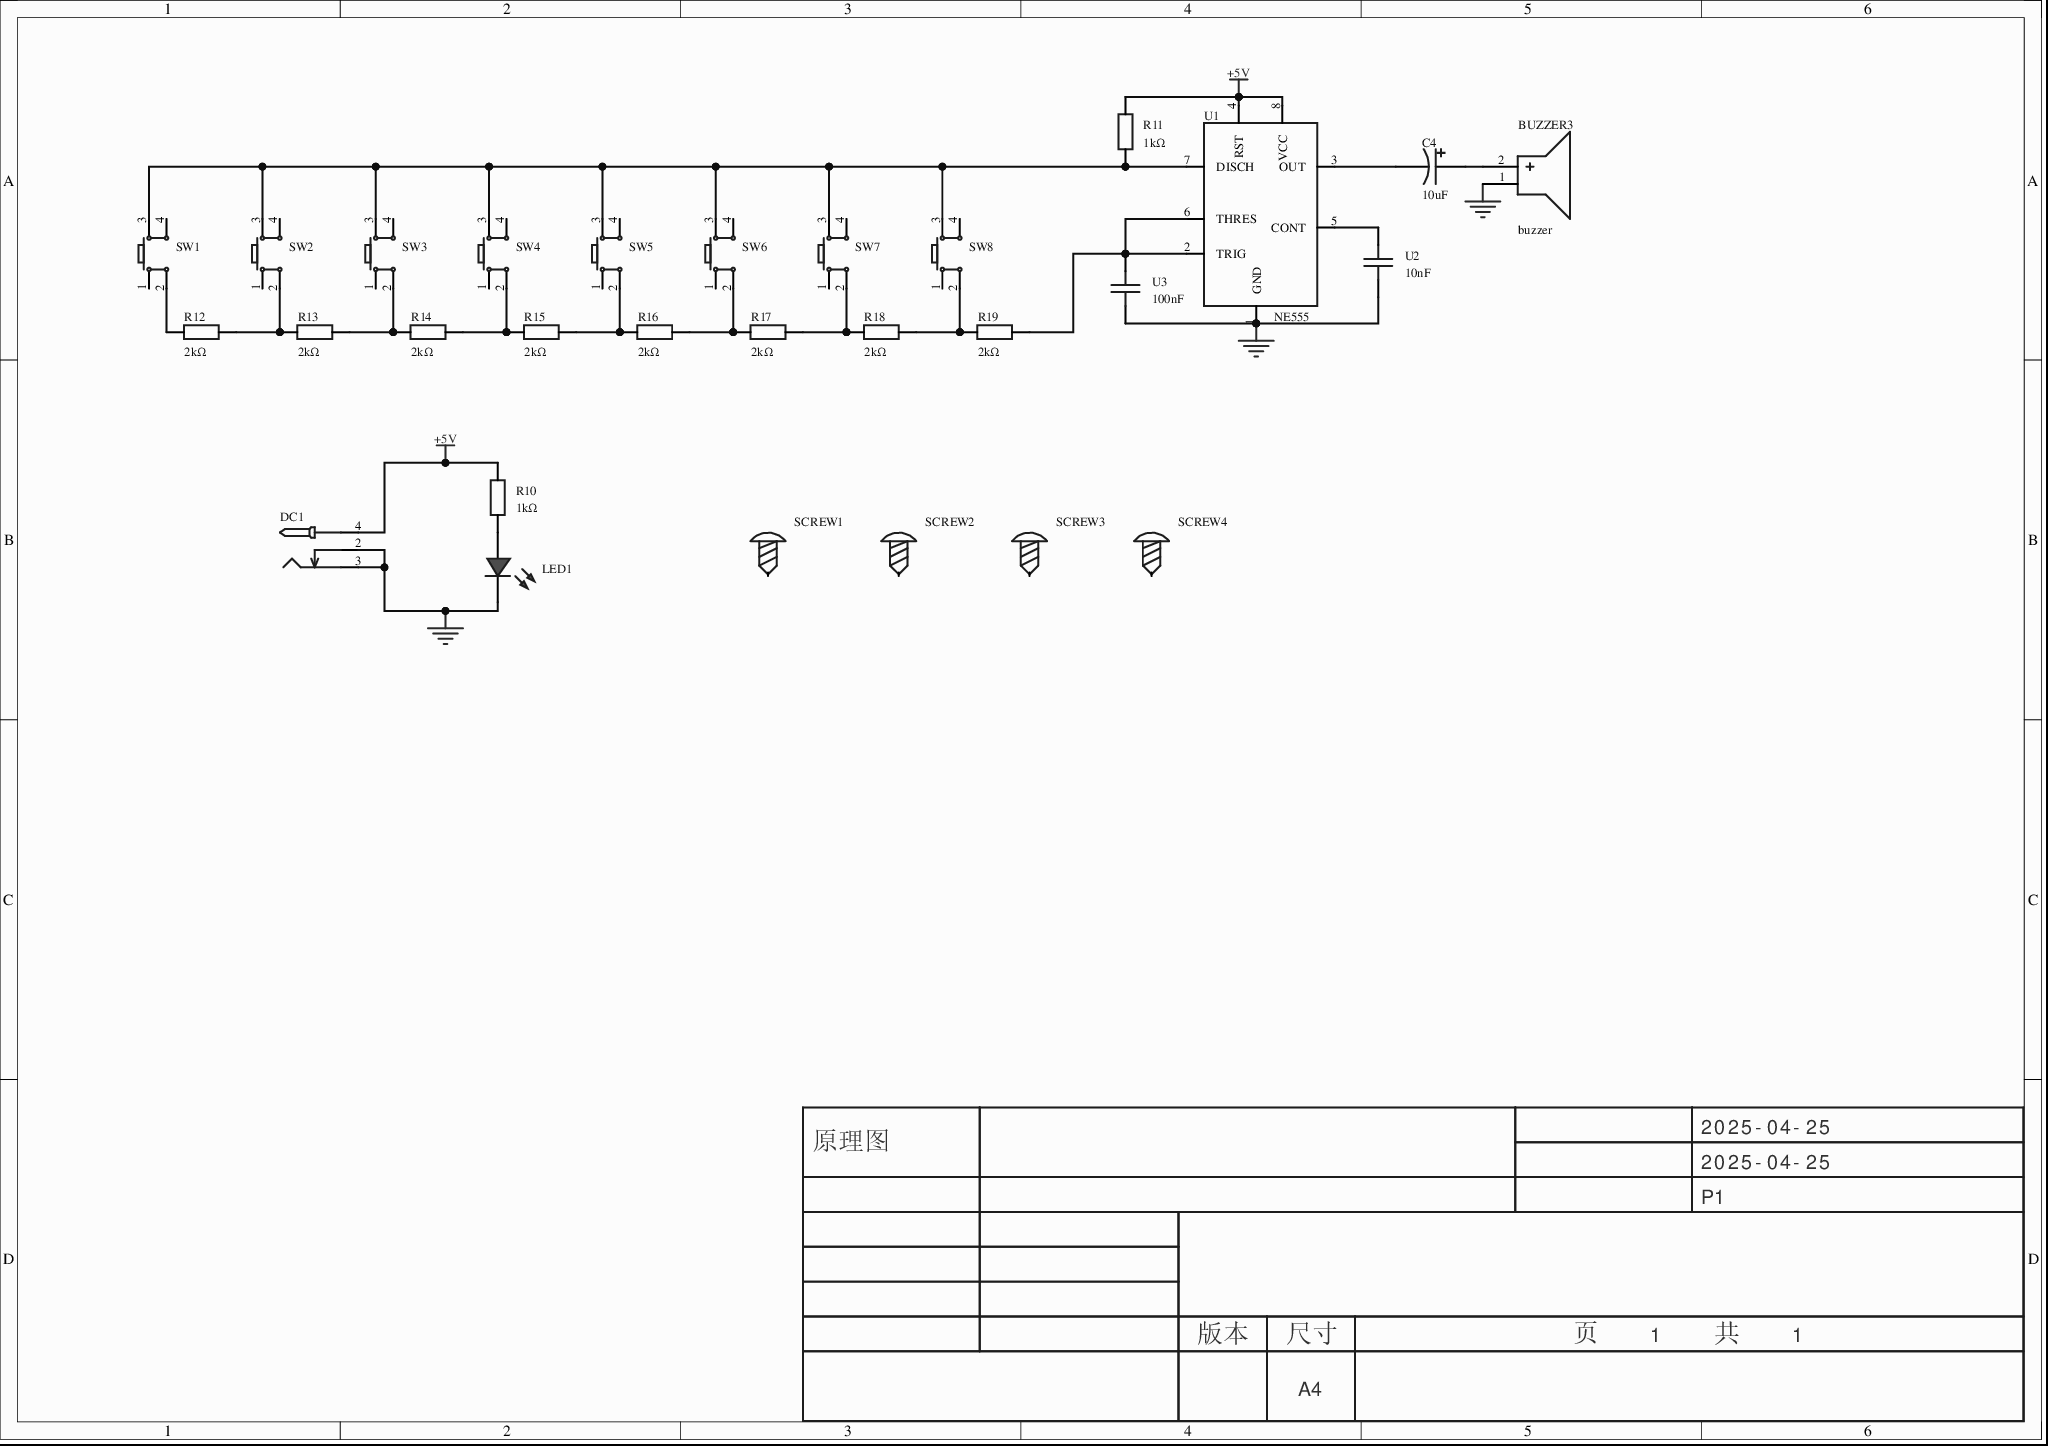
[diagram p0: MISC52051-3.schdoc]
# Altium project MISC52051-2.PrjPcb
1 sheet, 29 parts. Net scope: global (net labels, ports and power ports of the same name join across sheets).
Board file: MISC52051.pcbdoc

## Sheet MISC52051-3.schdoc
size 297 x 209 mm; Version: V1.0; @Project Name: MISC52051; @Page Count: 1; @Update Date: 2025-04-25; @Create Date: 2025-04-25; @Schematic Name: MISC52051; @Page No: 1; @Create Time: 16:50:07; @Update Time: 17:02:59; @Board Name: MISC52051

### Parts
BUZZER3  buzzer  [BUZ-TH_BD12.0-P6.00-D0.9-RD]
C4  10uF  [CAP-TH_BD5.0-P2.00-D0.8-FD]
DC1  (no value)  [DC-2.0]
LED1  (no value)  [LED_TH-3mm]
R10  1kΩ  [Res_1/8W]
R11  1kΩ  [Res_1/8W]
R12  2kΩ  [Res_1/8W]
R13  2kΩ  [Res_1/8W]
R14  2kΩ  [Res_1/8W]
R15  2kΩ  [Res_1/8W]
R16  2kΩ  [Res_1/8W]
R17  2kΩ  [Res_1/8W]
R18  2kΩ  [Res_1/8W]
R19  2kΩ  [Res_1/8W]
SCREW1  (no value)  [M3螺丝]
SCREW2  (no value)  [M3螺丝]
SCREW3  (no value)  [M3螺丝]
SCREW4  (no value)  [M3螺丝]
SW1  (no value)  [SW-TH_4P-L6.0-W6.0-P4.50-LS6.5]
SW2  (no value)  [SW-TH_4P-L6.0-W6.0-P4.50-LS6.5]
SW3  (no value)  [SW-TH_4P-L6.0-W6.0-P4.50-LS6.5]
SW4  (no value)  [SW-TH_4P-L6.0-W6.0-P4.50-LS6.5]
SW5  (no value)  [SW-TH_4P-L6.0-W6.0-P4.50-LS6.5]
SW6  (no value)  [SW-TH_4P-L6.0-W6.0-P4.50-LS6.5]
SW7  (no value)  [SW-TH_4P-L6.0-W6.0-P4.50-LS6.5]
SW8  (no value)  [SW-TH_4P-L6.0-W6.0-P4.50-LS6.5]
U1  NE555  [PDIP-8_L9.6-W6.4-P2.54-LS7.9-BL-1]
U2  10nF  [CAP-TH_L4.0-W2.5-P2.50-D0.5]
U3  100nF  [CAP-TH_L4.0-W2.5-P2.50-D0.5]

### Nets
+5V: DC1.4 R10.2 R11.2 U1.4(RST) U1.8(VCC)
GND: BUZZER3.1(-) DC1.2 DC1.3 LED1.2(A) U1.1(GND) U2.1 U3.1
NetBUZZER3_2: BUZZER3.2(+) C4.1
NetC4_2: C4.2 U1.3(OUT)
NetLED1_1: LED1.1(C) R10.1
NetR11_1: R11.1 SW1.3 SW2.3 SW3.3 SW4.3 SW5.3 SW6.3 SW7.3 SW8.3 U1.7(DISCH)
NetR12_1: R12.1 SW1.2
NetR12_2: R12.2 R13.1 SW2.2
NetR13_2: R13.2 R14.1 SW3.2
NetR14_2: R14.2 R15.1 SW4.2
NetR15_2: R15.2 R16.1 SW5.2
NetR16_2: R16.2 R17.1 SW6.2
NetR17_2: R17.2 R18.1 SW7.2
NetR18_2: R18.2 R19.1 SW8.2
NetR19_2: R19.2 U1.2(TRIG) U1.6(THRES) U3.2
NetU1_5: U1.5(CONT) U2.2

Not connected (* = marked no-connect by the designer): SCREW1 1; SCREW2 1; SCREW3 1; SCREW4 1; SW1 1 4; SW2 1 4; SW3 1 4; SW4 1 4; SW5 1 4; SW6 1 4; SW7 1 4; SW8 1 4

### Notes on the sheet
- 2025-04-25
- 原理图
- P1
- 版本
- 尺寸
- A4
- 页    1    共    1

### Library data of the parts
BUZZER3 = buzzer: AddInBom: yes; ModelId: af17e4151ed84fc2a628230bf2376363; ModelTransform: 472.44,472.176,0,270,0,0,0,0,-196.85; Symbol: BUZZER; Device: buzzer; LCSC Part Name: buzzer; SupplierPart: C9900014030; ManufacturerPart: buzzer; Supplier Footprint: buzzer; JLCPCB Part Class: 扩展库; Supplier: LCSC; ConvertToPcb: yes; FootprintName: BUZ-TH_BD12.0-P6.00-D0.9-RD; ModelName: BUZ-TH_BD12.0-P6.00-D0.9-RD
C4 = KM475M100D11RR0VH2FP0: 容值:4.7uF;精度:±20%;额定电压:100V;; Manufacturer: CX(承兴); Symbol: 4.7uF 100V 5*11; AddInBom: yes; ModelId: edeeed87cbc746108d01291548c38636; ModelName: CAP-TH_D5.0×H7.0×P2.0; ModelTransform: 197.091,196.7911,0,0,0,0,0,0,-137.795; Tolerance: ±20%; Rated Voltage: 100V; φD: 5mm; L: 11mm; Value: 10uF; Device: KM475M100D11RR0VH2FP0; LCSC Part Name: 4.7uF ±20% 100V; ManufacturerPart: KM475M100D11RR0VH2FP0; Supplier Footprint: 插件,D5xL11mm; JLCPCB Part Class: 扩展库; Datasheet: https://atta.szlcsc.com/upload/public/pdf/source/20211027/06D6BA3719C264B639DC286D935D03EA.pdf; Supplier: LCSC; ConvertToPcb: yes; FootprintName: CAP-TH_BD5.0-P2.00-D0.8-FD; Lead Spacing: 2mm; Lifetime @ Temp: -
DC1 = DC-005_2.0: ConvertToPcb: yes; SymbolName: DC电源接口; ModelId: f5f20b8a2308479b936ba3c2698865bb0819f05c4eef4c71ace90d822a990e87; ModelName: DC-IN-TH_DC-5520-1; ModelTransform: 372.05,551.18,582.68,90,0,0,137.8,0,-149.61; Device: DC-005_2.0; AddInBom: yes; Supplier Footprint: 插件; FootprintName: DC-2.0
LED1 = LED_TH-R_3mm: ConvertToPcb: yes; ModelId: a497c992633541038a38947cdc58012f; ModelName: LED-TH-3mm_R; ModelTransform: 141.274,153.327,0,0,0,0,-5.984,0,-137.795; Symbol: LED_TH-R; Device: LED_TH-R_3mm; AddInBom: yes; FootprintName: LED_TH-3mm; Supplier Footprint: 插件
R10-R19 = Res_AXIAL-1/8W: ConvertToPcb: yes; SymbolName: 电阻; ModelId: b2b5ae7ae4c642178fe0039925c86a3f; ModelName: RES-TH_BD1.8-L3.2-P7.20-D0.4; ModelTransform: 282.86,66.88,253.09,0,0,0,0,0,-191; Device: Res_AXIAL-1/8W; AddInBom: yes; Supplier Footprint: 轴向引线; FootprintName: Res_1/8W
  R10 R11: Value: 1kΩ
  R12-R19: Value: 2kΩ
SCREW1-SCREW4 = M3螺丝: ConvertToPcb: yes; SymbolName: 螺丝孔; Device: M3螺丝; AddInBom: yes; Supplier Footprint: 插件; FootprintName: M3螺丝
SW1-SW8 = Key_TH_6x6x6: 触点电流:50mA;额定电压(DC):12V;绝缘电阻:100MΩ;电路结构:单刀单掷;安装方式:直插;按钮形状:圆形按钮;按钮/盖帽颜色:黑色;作用力:260gf@±30gf;工作温度:-25℃~+70℃;引脚样式:PC引脚;开关长度:6mm;开关宽度:6mm;开关高度:6mm;带支架:否;; Symbol: 轻触按键; ConvertToPcb: yes; ModelId: 20eee248bc684ccd8cbdbb1d0d91ec6f; ModelName: SW-TH_4P-L6.0-W6.0-H5.0-LS6.5-P4.50; ModelTransform: 236.22,323.03,0,90,0,0,0,0,-137.795; Device: Key_TH_6x6x6; AddInBom: yes; SupplierPart: C2837516; Supplier Footprint: 插件; FootprintName: SW-TH_4P-L6.0-W6.0-P4.50-LS6.5
U1 = NE555PE4: NE555 单精度定时器; Manufacturer: TI(德州仪器); AddInBom: yes; ModelId: 1b8eaf096e7944deafe216467068c10e; ModelTransform: 377.952,318.897,0,0,0,0,0,0,-118.11; Manufacturer Part: NE555; Symbol: NE555PE4; Device: NE555PE4; LCSC Part Name: NE555PE4; SupplierPart: C2859604; Supplier Footprint: PDIP-8; JLCPCB Part Class: 扩展库; Datasheet: https://www.ti.com/cn/lit/gpn/sa555; Supplier: LCSC; ConvertToPcb: yes; FootprintName: PDIP-8_L9.6-W6.4-P2.54-LS7.9-BL-1; ModelName: PDIP-8_L9.6-W6.4-P2.54-LS7.9-BL-1
U2 U3 = FK18X7R1H103K: 容值:10nF;精度:±10%;额定电压:50V;温度系数:X7R;; Manufacturer: TDK; AddInBom: yes; ModelId: 29f34a7a495a447ab8bf96a7f673455e; ModelTransform: 189.7897,98.8187,0,0,0,0,0,0,-196.85; Tolerance: ±10%; Voltage Rated: 50V; Temperature Coefficient: X7R; Symbol: FK18X7R1H103K; Device: FK18X7R1H103K; LCSC Part Name: 10nF ±10% 50V; ManufacturerPart: FK18X7R1H103K; Supplier Footprint: -; JLCPCB Part Class: 扩展库; Supplier: LCSC; ConvertToPcb: yes; FootprintName: CAP-TH_L4.0-W2.5-P2.50-D0.5; ModelName: CAP-TH_L4.0-W2.5-P2.50-D0.5
  U2: SupplierPart: C3690803; Value: 10nF
  U3: Value: 100nF